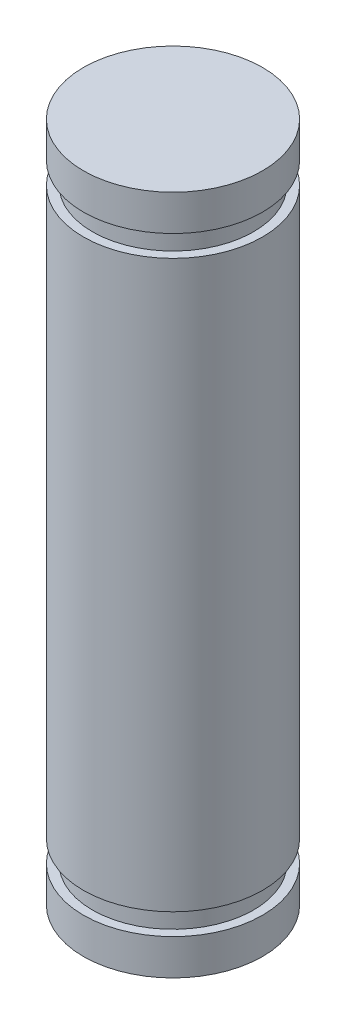
from build123d import *


with BuildPart() as part:
    # 草图1 → 旋转1 (revolve)
    with BuildSketch(Plane(origin=(0, 0, 0), x_dir=(-1, 0, 0), z_dir=(0, 0, -1)), mode=Mode.PRIVATE) as revolve_1_sk:
        Polygon((-5, -19), (0, -19), (0, 19), (-5, 19), (-5, 17), (-4.5, 17), (-4.5, 15.8), (-5, 15.8), (-5, -15.8), (-4.5, -15.8), (-4.5, -17), (-5, -17), align=None)
    revolve(revolve_1_sk.sketch.rotate(Axis((0, -19, 0), (0, 1, 0)), 270), axis=Axis((0, -19, 0), (0, 1, 0)))


solid = part.part
